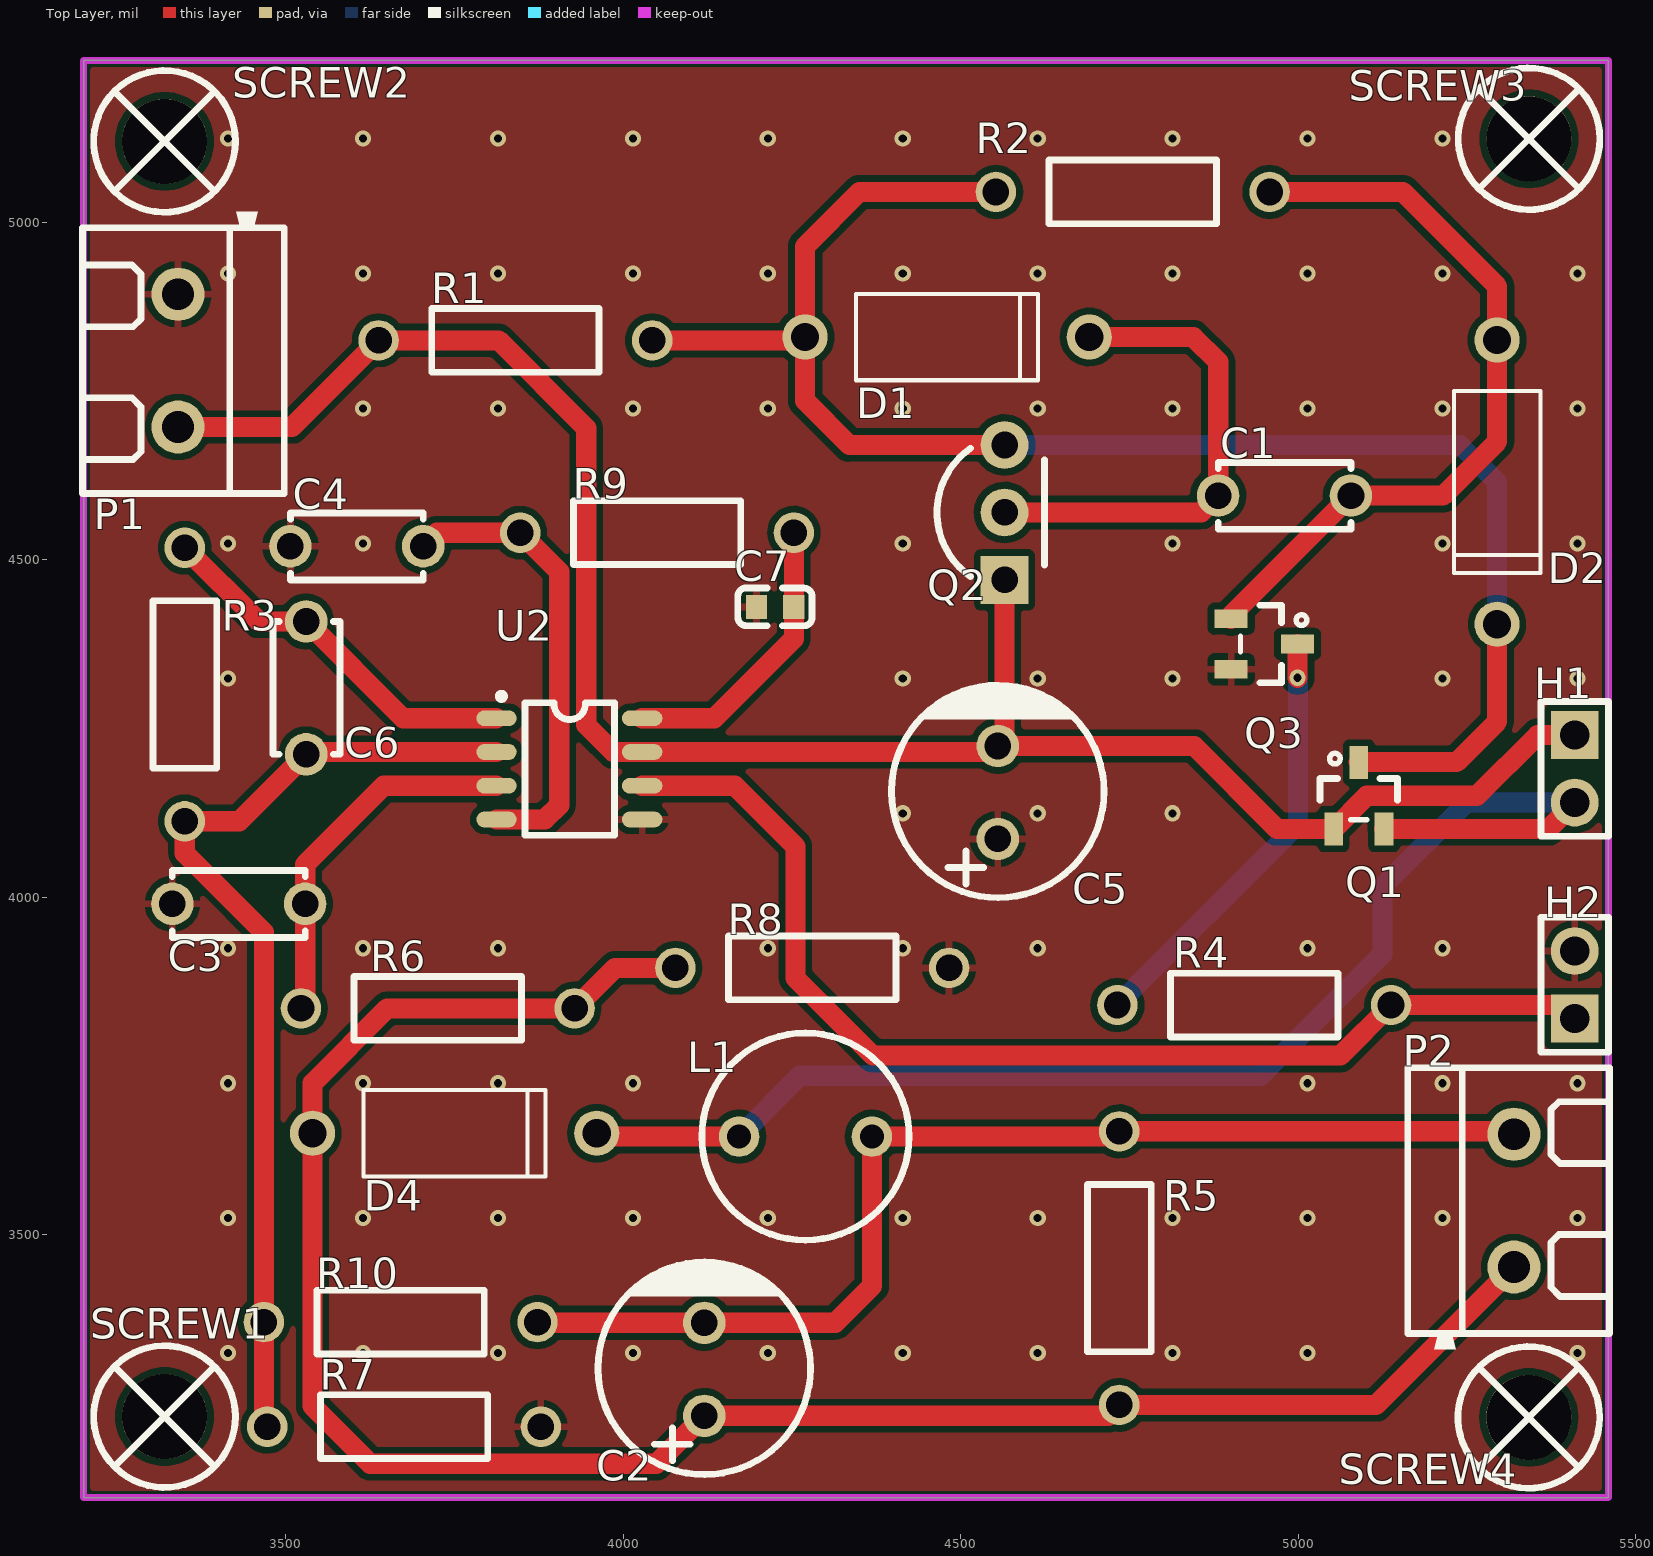
[diagram p0: Top Layer view]
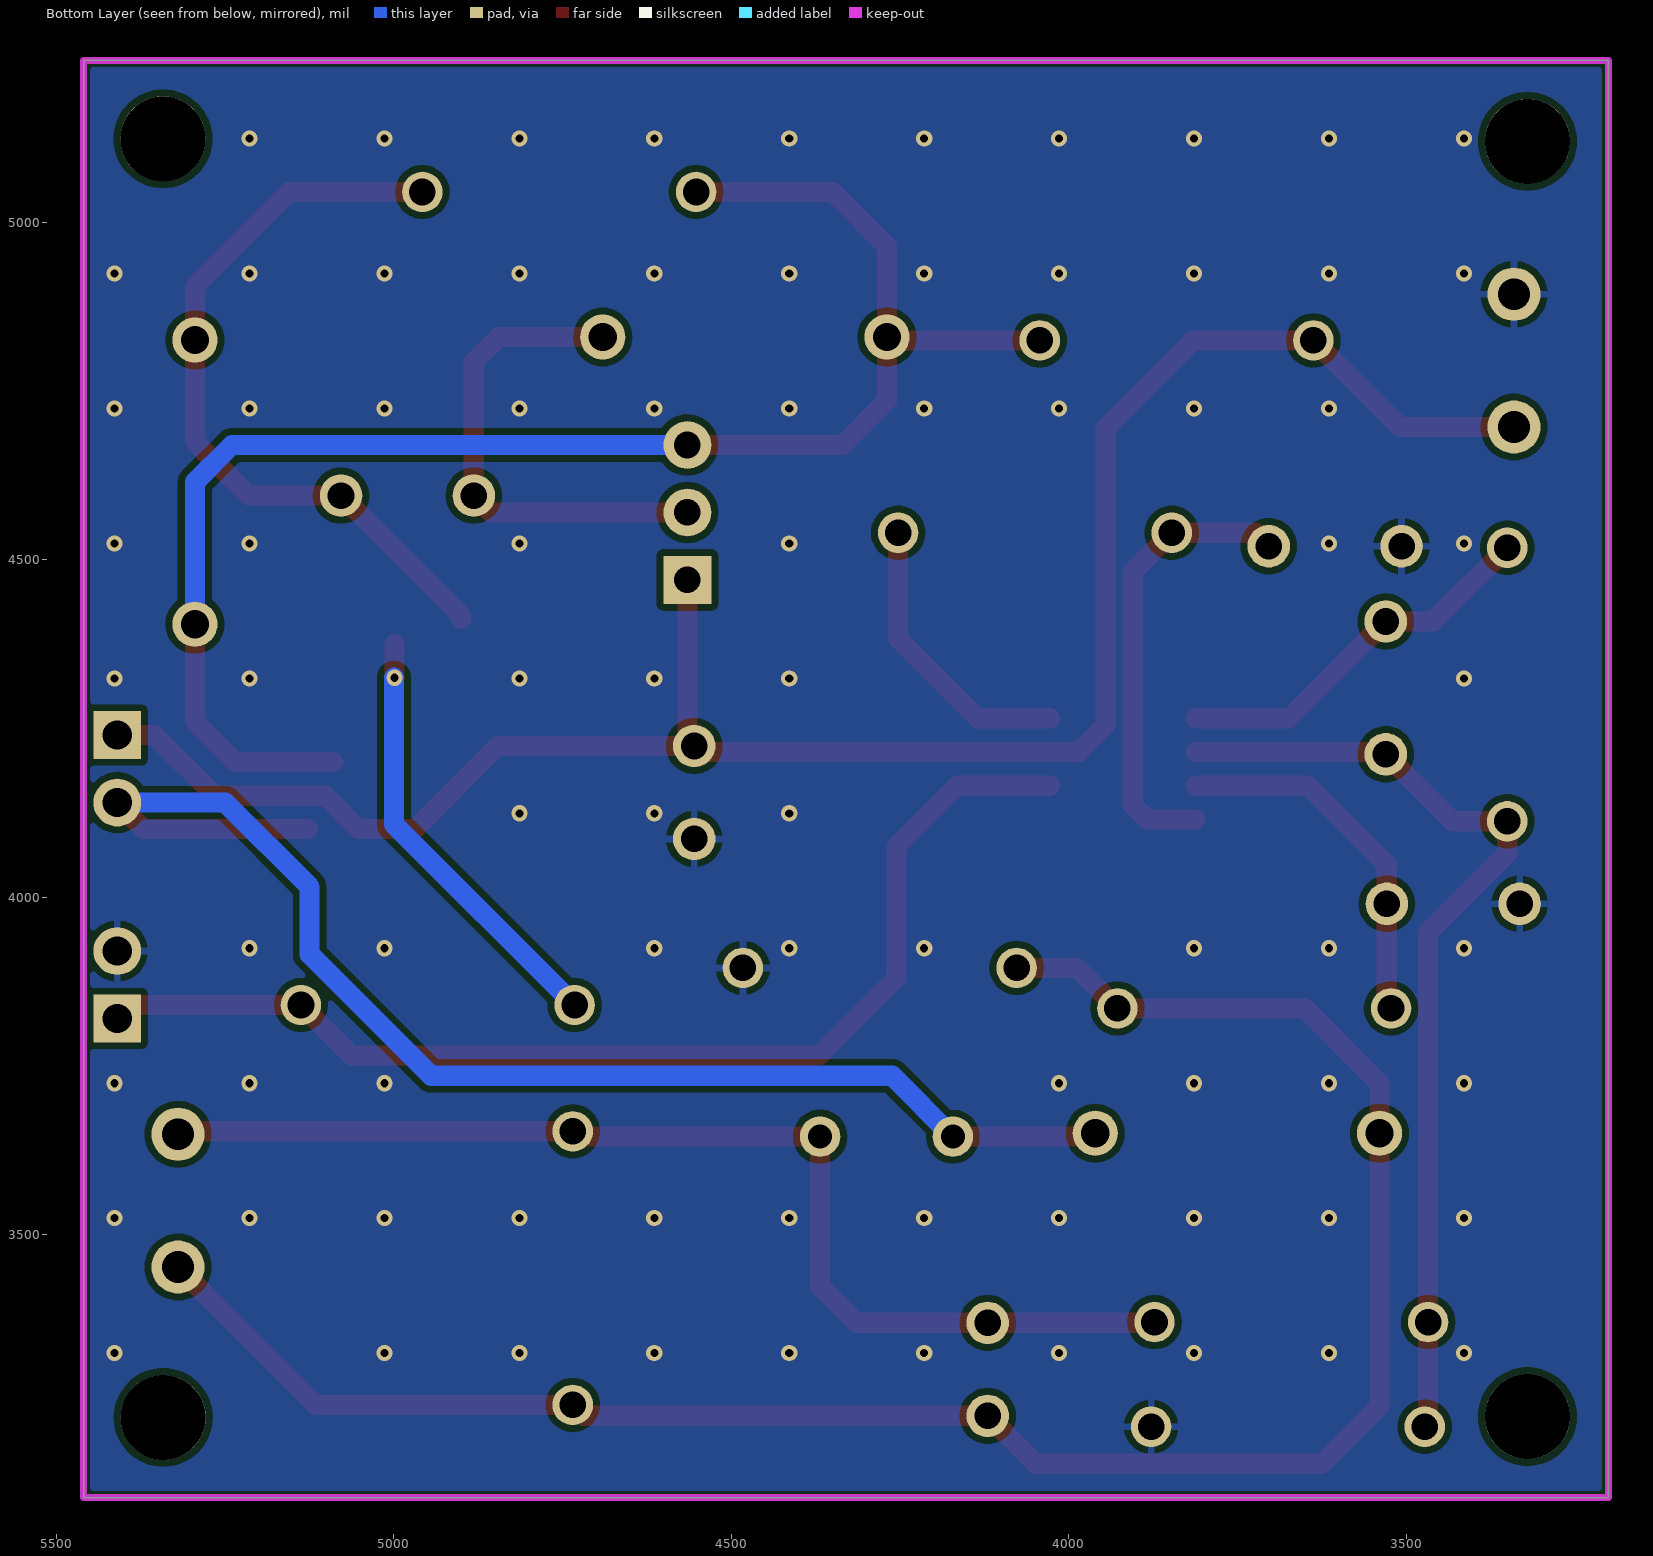
[diagram p1: Bottom Layer view, seen from below]
# Altium PCB MISC50807.pcbdoc
Units mil, origin at the board's own origin, x right, y up, seen from the top; angles counter-clockwise.
Board outline 2260 x 2130 mil, 2 copper layers (Top Layer, Bottom Layer), stack 62.206 mil thick; 33 components, 15 nets, 71 pads, 83 vias.

## Layer stack, top to bottom
Top Solder Mask Layer: solder mask 0.394, Dk 3.3
Top Layer: signal copper 1.379
Dielectric1: surface 59.449, FR4, Dk 4.5
Bottom Layer: signal copper 1.378
Bottom Solder Mask Layer: solder mask 0.394, Dk 3.3

## Board outline
3200,5240 3200,3110 5460,3110 5460,5240

## Design rules (kind name [scope] priority, off if disabled: settings)
BoardOutlineClearance copperThickness2oz_1 [All] p2 off: genericclearance=7.99 ignorepadtopadclearanceinfootprint=FALSE except(0: Arc-SplitContinuation Track-SplitContinuation SMDPad-SplitContinuation THPad-SplitContinuation Via-SplitContinuation Fill-SplitContinuation Region-SplitContinuation Poly-SplitContinuation Text-SplitContinuation Hole-SplitContinuation; 5.98: Arc-CutoutEdge SMDPad-CutoutEdge THPad-CutoutEdge Via-CutoutEdge Fill-CutoutEdge Region-CutoutEdge Text-CutoutEdge; 6.93: Hole-OutlineEdge Hole-CutoutEdge; 10: Poly-OutlineEdge Poly-CutoutEdge; 11.81: Arc-OutlineEdge Track-OutlineEdge SMDPad-OutlineEdge THPad-OutlineEdge Via-OutlineEdge Fill-OutlineEdge Region-OutlineEdge Text-OutlineEdge Track-CutoutEdge)
BoardOutlineClearance Plane_innerPlane_1 [All] p4 off: genericclearance=4.02 ignorepadtopadclearanceinfootprint=FALSE except(0: Arc-SplitContinuation Track-SplitContinuation SMDPad-SplitContinuation THPad-SplitContinuation Via-SplitContinuation Fill-SplitContinuation Region-SplitContinuation Poly-SplitContinuation Text-SplitContinuation Hole-SplitContinuation; 6: SMDPad-CutoutEdge THPad-CutoutEdge Via-CutoutEdge Fill-CutoutEdge Region-CutoutEdge Text-CutoutEdge; 6.93: Hole-OutlineEdge Hole-CutoutEdge; 10: Poly-OutlineEdge Poly-CutoutEdge; 11.8: Arc-OutlineEdge Track-OutlineEdge SMDPad-OutlineEdge THPad-OutlineEdge Via-OutlineEdge Fill-OutlineEdge Region-OutlineEdge Text-OutlineEdge; 11.81: Arc-CutoutEdge Track-CutoutEdge)
BoardOutlineClearance Copper_copperRegion_1 [All] p6 off: genericclearance=4.02 ignorepadtopadclearanceinfootprint=FALSE except(0: Arc-SplitContinuation Track-SplitContinuation SMDPad-SplitContinuation THPad-SplitContinuation Via-SplitContinuation Fill-SplitContinuation Region-SplitContinuation Poly-SplitContinuation Text-SplitContinuation Hole-SplitContinuation; 6: SMDPad-CutoutEdge THPad-CutoutEdge Via-CutoutEdge Fill-CutoutEdge Region-CutoutEdge Text-CutoutEdge; 6.93: Hole-OutlineEdge Hole-CutoutEdge; 10: Poly-OutlineEdge Poly-CutoutEdge; 11.8: Arc-OutlineEdge Track-OutlineEdge SMDPad-OutlineEdge THPad-OutlineEdge Via-OutlineEdge Fill-OutlineEdge Region-OutlineEdge Text-OutlineEdge; 11.81: Arc-CutoutEdge Track-CutoutEdge)
BoardOutlineClearance copperThickness1oz_1 [All] p8: genericclearance=4.02 ignorepadtopadclearanceinfootprint=FALSE except(0: Arc-SplitContinuation Track-SplitContinuation SMDPad-SplitContinuation THPad-SplitContinuation Via-SplitContinuation Fill-SplitContinuation Region-SplitContinuation Poly-SplitContinuation Text-SplitContinuation Hole-SplitContinuation; 6: SMDPad-CutoutEdge THPad-CutoutEdge Via-CutoutEdge Fill-CutoutEdge Region-CutoutEdge Text-CutoutEdge; 6.93: Hole-OutlineEdge Hole-CutoutEdge; 10: Poly-OutlineEdge Poly-CutoutEdge; 11.8: Arc-OutlineEdge Track-OutlineEdge SMDPad-OutlineEdge THPad-OutlineEdge Via-OutlineEdge Fill-OutlineEdge Region-OutlineEdge Text-OutlineEdge; 11.81: Arc-CutoutEdge Track-CutoutEdge)
Clearance copperThickness2oz [All] p1 off: gap=7.99 ignorepadtopadclearanceinfootprint=FALSE except(5.98: SMDPad-Track SMDPad-SMDPad THPad-Track SMDPad-THPad THPad-THPad Track-Via SMDPad-Via THPad-Via Via-Via Fill-Track Region-Track Fill-SMDPad Region-SMDPad Fill-THPad Region-THPad Fill-Via Region-Via Fill-Fill Fill-Region Region-Region Arc-Track Arc-SMDPad Arc-THPad Arc-Via Fill-Arc Region-Arc Arc-Arc Text-Track SMDPad-Text Text-THPad Text-Via Fill-Text Region-Text Arc-Text Text-Text; 6.93: Hole-Track Hole-SMDPad Hole-THPad Hole-Via Fill-Hole Region-Hole Hole-Arc Hole-Text; 10: Poly-Track Poly-SMDPad Poly-THPad Poly-Via Poly-Fill Poly-Region Poly-Poly Poly-Arc Poly-Text Poly-Hole)
Clearance Plane_innerPlane [All] p3 off: gap=4.02 ignorepadtopadclearanceinfootprint=FALSE except(5.98: SMDPad-Track SMDPad-SMDPad THPad-Track SMDPad-THPad THPad-THPad Track-Via SMDPad-Via THPad-Via Via-Via Fill-Track Region-Track Fill-SMDPad Region-SMDPad Fill-THPad Region-THPad Fill-Via Region-Via Fill-Fill Fill-Region Region-Region; 6: Arc-Track Arc-SMDPad Arc-THPad Arc-Via Fill-Arc Region-Arc Arc-Arc Text-Track SMDPad-Text Text-THPad Text-Via Fill-Text Region-Text Arc-Text Text-Text; 6.93: Hole-Track Hole-SMDPad Hole-THPad Hole-Via Fill-Hole Region-Hole Hole-Arc Hole-Text; 10: Poly-Track Poly-SMDPad Poly-THPad Poly-Via Poly-Fill Poly-Region Poly-Poly Poly-Arc Poly-Text Poly-Hole)
Clearance Copper_copperRegion [All] p5 off: gap=4.02 ignorepadtopadclearanceinfootprint=FALSE except(5.98: SMDPad-Track SMDPad-SMDPad THPad-Track SMDPad-THPad THPad-THPad Track-Via SMDPad-Via THPad-Via Via-Via Fill-Track Region-Track Fill-SMDPad Region-SMDPad Fill-THPad Region-THPad Fill-Via Region-Via Fill-Fill Fill-Region Region-Region; 6: Arc-Track Arc-SMDPad Arc-THPad Arc-Via Fill-Arc Region-Arc Arc-Arc Text-Track SMDPad-Text Text-THPad Text-Via Fill-Text Region-Text Arc-Text Text-Text; 6.93: Hole-Track Hole-SMDPad Hole-THPad Hole-Via Fill-Hole Region-Hole Hole-Arc Hole-Text; 10: Poly-Track Poly-SMDPad Poly-THPad Poly-Via Poly-Fill Poly-Region Poly-Poly Poly-Arc Poly-Text Poly-Hole)
Clearance copperThickness1oz [All] p7: gap=4.02 ignorepadtopadclearanceinfootprint=FALSE except(5.98: SMDPad-Track SMDPad-SMDPad THPad-Track SMDPad-THPad THPad-THPad Track-Via SMDPad-Via THPad-Via Via-Via Fill-Track Region-Track Fill-SMDPad Region-SMDPad Fill-THPad Region-THPad Fill-Via Region-Via Fill-Fill Fill-Region Region-Region; 6: Arc-Track Arc-SMDPad Arc-THPad Arc-Via Fill-Arc Region-Arc Arc-Arc Text-Track SMDPad-Text Text-THPad Text-Via Fill-Text Region-Text Arc-Text Text-Text; 6.93: Hole-Track Hole-SMDPad Hole-THPad Hole-Via Fill-Hole Region-Hole Hole-Arc Hole-Text; 10: Poly-Track Poly-SMDPad Poly-THPad Poly-Via Poly-Fill Poly-Region Poly-Poly Poly-Arc Poly-Text Poly-Hole)
DiffPairsRouting differentialPair [All] p1: maxlimit=6 minlimit=6 mostfreqgap=6 toplayer_minwidth=5 toplayer_prefwidth=10 toplayer_maxwidth=100 toplayer_mingap=6 toplayer_prefgap=6 toplayer_maxgap=6 bottomlayer_minwidth=5 bottomlayer_prefwidth=10 bottomlayer_maxwidth=100 bottomlayer_mingap=6 bottomlayer_prefgap=6 bottomlayer_maxgap=6 maxuncoupledlength=10
HoleToHoleClearance otherClearance [All] p1: gap=11.81 allowstackedmicrovias=TRUE
Length netLength [All] p1: minlimit=0 maxlimit=0
PasteMaskExpansion pasteMaskExpansion [All] p1: expansion=0
PlaneConnect innerPlane [All] p1: planeconnectstyle=Relief reliefexpansion=20 reliefentries=4 reliefconductorwidth=10 reliefairgap=10
PolygonConnect copperRegion [All] p1: connectstyle=Relief reliefconductorwidth=10 reliefentries=4 polygonreliefangle="90 Angle" airgapwidth=10 via.connectstyle=Relief via.reliefconductorwidth=10 via.reliefentries=4 via.polygonreliefangle="90 Angle" via.airgapwidth=10
RoutingVias viaSize [All] p1: holewidth=12.01 width=24.02 viastyle="Through Hole" minholewidth=11.81 minwidth=19.68 maxholewidth=248.03 maxwidth=393.7
SolderMaskExpansion solderMaskExpansion [IsVia] p1: expansion=-1000 istentingtop=TRUE
SolderMaskExpansion solderMaskExpansion [All] p2: expansion=2 istentingtop=FALSE
Width copperThickness2oz_2 [All] p1 off: maxlimit=100 minlimit=8 preferedwidth=10
Width copperThickness1oz_2 [All] p2: maxlimit=100 minlimit=5 preferedwidth=10

## Components (designator, comment, footprint, x,y, rotation, side; value= is the part's Value field where it differs from the comment)
C1 "1000pF" CAP-TH_L5.0-W2.5-P5.00-D1.0 4980,4595 r0 top
C2 "100uF" CAP-TH_BD8.0-P3.50-D0.6-FD_1 4120,3300 r90 top
C3 "470pF" CAP-TH_L5.0-W2.5-P5.00-D1.0 3430,3990 r0 top
C4 "4.7nF" CAP-TH_L5.0-W2.5-P5.00-D1.0 3605,4520 r0 top
C5 "100uF" CAP-TH_BD8.0-P3.50-D0.6-FD_1 4555,4155 r90 top
C6 "10nF" CAP-TH_L5.0-W2.5-P5.00-D1.0 3530,4310 r90 top
C7 "10nF" C0603 4225,4430 r0 top
D1 "SS34" DO-15_BD3.1-L6.7-P10.70-D0.8-RD 4480,4830 r180 top
D2 "1N5341BRLG" DO-15_BD3.1-L6.7-P10.70-D0.8-RD 5295,4615 r90 top
D4 "SS34" DO-15_BD3.1-L6.7-P10.70-D0.8-RD 3750,3650 r180 top
H1 "" HDR-TH_2P-P2.54-V-M-1 5410,4190 r270 top
H2 "" HDR-TH_2P-P2.54-V-M-1 5410,3870 r90 top
L1 "33uH" IND-TH_BD7.8-P5.00-D0.7 4270,3645 r0 top
P1 "KF301-2P terminal block" CONN-TH_XY301V-A-5.0-2P 3340,4795 r90 top
P2 "KF301-2P terminal block" CONN-TH_XY301V-A-5.0-2P 5320,3550 r270 top
Q1 "AOD4185" SOT-23-3_L2.9-W1.3-P1.90-LS2.4-L 5090,4150 r270 top
Q2 "BC33725TA" TO-92-3_L4.9-W3.7-P2.54-L 4565,4570 r90 top
Q3 "SI2302DS" SOT-23-3_L2.9-W1.3-P1.90-LS2.4-L 4950,4375 r180 top
R1 "300" Res_1/4W 3840,4825 r0 top
R2 "200" Res_1/4W 4755,5045 r0 top
R3 "4.7K" Res_1/4W 3350,4315 r90 top
R4 "10" Res_1/4W 4935,3840 r0 top
R5 "2.5" Res_1/4W 4735,3450 r90 top
R6 "1K" Res_1/4W 3725,3835 r0 top
R7 "2.5K" Res_1/4W 3675,3215 r180 top
R8 "0.1" Res_1/4W 4280,3895 r180 top
R9 "2K" Res_1/4W 4050,4540 r0 top
R10 "2.5K" Res_1/4W 3670,3370 r0 top
SCREW1 "" M3螺丝 3320,3230 r0 top
SCREW2 "" M3螺丝 3320,5120 r0 top
SCREW3 "" M3螺丝 5342.32,5123.78 r0 top
SCREW4 "" M3螺丝 5342.01,3228.78 r0 top
U2 "UC3843N" SOP-8_L5.1-W3.9-P1.27-LS6.0-BL 3920,4190 r270 top

## Footprints (in the part's own frame and the unit in brackets; to place one, negate y for a bottom-side part, rotate by r counter-clockwise, add the part's x,y. Pads: shape width x height; smd on the part's side, far side on the other; paste and mask are expansions set on the pad)
C0603 [mm]
  rect 0.8x0.9 smd: 1(-0.7,0) 2(0.7,0)
  silkscreen extent -1.41,-0.71 1.39,0.72
CAP-TH_BD8.0-P3.50-D0.6-FD_1 [mm]
  round 1.6 hole 1: 1(-1.75,0) 2(1.75,0)
  silkscreen extent -3.96,-4 4.04,4
CAP-TH_L5.0-W2.5-P5.00-D1.0 [mm]
  round 1.6 hole 1: 1(-2.5,0) 2(2.5,0)
  silkscreen extent -2.5,-1.27 2.5,1.25
CONN-TH_XY301V-A-5.0-2P [mm]
  round 2 hole 1.2: 1(-2.5,0) 2(2.5,0)
  silkscreen extent -5,-4 5.6,3.6
DO-15_BD3.1-L6.7-P10.70-D0.8-RD [mm]
  round 1.7 hole 1.06: 1(-5.35,0) 2(5.35,0)
  silkscreen extent -3.43,-1.63 3.43,1.63
HDR-TH_2P-P2.54-V-M-1 [mm]
  rect 1.8x1.8 hole 1.1: 1(-1.27,0)
  round 1.8 hole 1.1: 2(1.27,0)
  silkscreen extent -2.54,-1.27 2.54,1.27
IND-TH_BD7.8-P5.00-D0.7 [mil]
  round 60 hole 36: 1(-98.43,0) 2(98.42,0)
  silkscreen extent -154,-154 154,154
M3螺丝 [mil]
  round 126 hole 126 paste+0 mask+4: 1(0,0)
  silkscreen extent -105,-105 105,105
Res_1/4W [mil]
  round 60 hole 39.37 paste+0 mask+2: 1(-202.76,0) 2(202.76,0)
  silkscreen extent -124,-47 124,47
SOP-8_L5.1-W3.9-P1.27-LS6.0-BL [mm]
  oval 0.6x1.52 smd: 1(-1.905,-2.74) 2(-0.635,-2.74) 3(0.635,-2.74) 4(1.905,-2.74) 5(1.905,2.74) 6(0.635,2.74) 7(-0.635,2.74) 8(-1.905,2.74)
  silkscreen extent -2.85,-2.68 2.5,1.7
SOT-23-3_L2.9-W1.3-P1.90-LS2.4-L [mm]
  rect 1.25x0.7 smd: 1(-1.25,0) 2(1.25,0.95) 3(1.25,-0.95)
  silkscreen extent -1.6,-1.46 0.9,1.46
TO-92-3_L4.9-W3.7-P2.54-L [mm]
  rect 1.8x1.8 hole 1: 1(-2.54,0)
  round 1.8 hole 1: 2(0,0) 3(2.54,0)
  silkscreen extent -2.41,-1.5 2.41,2.54

## Via types
v1: diameter 24.02, hole 12, Top Layer to Bottom Layer, 83 vias

## Nets (pads, with @x,y where several pads share a name; then routed paths per layer and width w, separated by ;. In a path a pad name is that pad's centre, name@x,y a point inside that pad or via, vN(x,y) a via of type N, cw(c..) or ccw(c..) an arc to the next point about the centre after c; other vN are vias at no path point)
$1N5: C1.2 D2.2 Q3.3 R2.2 | length 1131.1
  Top Layer w30: Q3.3 4900.8,4417.38 C1.2 5215,4595 5295,4675 D2.2 5295,4905 5155,5045 R2.2
$1N6: C1.1 D1.1 Q2.2 | length 731.5
  Top Layer w30: Q2.2 4856.57,4570 C1.1 4881.57,4793.43 4845,4830 D1.1
$1N12: C2.1 D4.2 P2.2 R5.1 R6.2 R8.2 | length 3024.2
  Top Layer w30: R8.2 3987.76,3895 R6.2 3650,3835 3539.37,3724.37 D4.2 3539.37,3245.63 3625,3160 4048.9,3160 C2.1 4718.86,3231.1 R5.1 5115.66,3247.24 P2.2
$1N13: C2.2 L1.2 P2.1 R5.2 R10.2 | length 1696.9
  Top Layer w30: R10.2 3873.86,3368.9 C2.2 4313.9,3368.9 4368.43,3423.43 L1.2 4727.24,3645 R5.2 5315.66,3652.76 P2.1
$1N14: C6.1 R3.1 R7.2 R10.1 U2.2 | length 1452.6
  Top Layer w30: R7.2 3467.24,3220 R10.1 3467.24,3947.76 3350,4065 R3.1 3430.66,4112.24 C6.1 3533.42,4215 U2.2
$1N15: C6.2 R3.2 U2.1 | length 566.8
  Top Layer w30: R3.2 3459.34,4408.43 C6.2 3673.43,4265 U2.1
$1N18: C4.2 R9.1 U2.4 | length 681.5
  Top Layer w30: C4.2 3723.43,4540 R9.1 3905,4482.24 3905,4136.21 3883.79,4115 U2.4
$1N19: C7.2 R9.2 U2.8 | length 430.9
  Top Layer w30: U2.8 4135,4265 4252.76,4382.76 R9.2
$1N20: C3.2 R6.1 U2.3 | length 548
  Top Layer w30: R6.1 3528.43,3841.18 C3.2 3528.43,4048.43 3645,4165 U2.3
$1N23: D1.2 D2.1 Q1.1 Q2.3 R1.2 R2.1 | length 2434.1
  Top Layer w30: R1.2 4264.37,4825 D1.2 ; R2.1 4350,5045 4269.37,4964.37 D1.2 ; Q2.3 4335,4670 4269.37,4735.63 D1.2 ; Q1.1@5090,4200 5235,4200 5295,4260 D2.1
  Bottom Layer w30: Q2.3 5240,4670 5295,4615 D2.1
$1N24: D4.1 H1.2 L1.1 Q1.2 | length 2013.9
  Top Layer w30: D4.1 3965.63,3645 L1.1 ; Q1.2 5370.8,4100.8 H1.2
  Bottom Layer w30: L1.1 4261.57,3735 4945,3735 5125,3915 5125,4015 5250,4140 H1.2
$1N27: Q3.1 R4.1 | length 645.9
  Top Layer w30: v1(4999.2,4325) Q3.1
  Bottom Layer w30: R4.1 5000,4107.76 v1@5000,4325
$1N28: H2.1 R4.2 U2.6 | length 1701.4
  Top Layer w30: U2.6 4165,4165 4255,4075 4255,3880 4370,3765 5062.76,3765 R4.2 5390,3840 H2.1
+15V: C5.2 H1.1 P1.1 Q1.3 Q2.1 R1.1 U2.7 | length 2996.2
  Top Layer w30: P1.1 3508.82,4696.57 R1.1 3815,4825 3945,4695 3945,4255 3985,4215 U2.7 4546.1,4215 C5.2 ; Q2.1 4565,4233.9 C5.2 ; H1.1 5355,4240 5265,4150 5101.8,4150 Q1.3 4969.2,4100.8 4846.1,4223.9 C5.2
GND: C3.1 C4.1 C5.1 C7.1 H2.2 P1.2 Q3.2 R7.1 R8.1 U2.5
  other v1: 3414.1,3324.1 3614.1,3324.1 3814.1,3324.1 4014.1,3324.1 4214.1,3324.1 4414.1,3324.1 4614.1,3324.1 4814.1,3324.1 5014.1,3324.1 5414.1,3324.1 3414.1,3524.1 3614.1,3524.1 3814.1,3524.1 4014.1,3524.1 4214.1,3524.1 4414.1,3524.1 4614.1,3524.1 4814.1,3524.1 5014.1,3524.1 5214.1,3524.1 5414.1,3524.1 3414.1,3724.1 3614.1,3724.1 3814.1,3724.1 4014.1,3724.1 5014.1,3724.1 5214.1,3724.1 5414.1,3724.1 3414.1,3924.1 3614.1,3924.1 3814.1,3924.1 4214.1,3924.1 4414.1,3924.1 4614.1,3924.1 5014.1,3924.1 5214.1,3924.1 4414.1,4124.1 4614.1,4124.1 4814.1,4124.1 3414.1,4324.1 4414.1,4324.1 4614.1,4324.1 4814.1,4324.1 5214.1,4324.1 5414.1,4324.1 3414.1,4524.1 3614.1,4524.1 4414.1,4524.1 4814.1,4524.1 5214.1,4524.1 5414.1,4524.1 3614.1,4724.1 3814.1,4724.1 4014.1,4724.1 4214.1,4724.1 4414.1,4724.1 4614.1,4724.1 4814.1,4724.1 5014.1,4724.1 5214.1,4724.1 5414.1,4724.1 3414.1,4924.1 3614.1,4924.1 3814.1,4924.1 4014.1,4924.1 4214.1,4924.1 4414.1,4924.1 4614.1,4924.1 4814.1,4924.1 5014.1,4924.1 5214.1,4924.1 5414.1,4924.1 3414.1,5124.1 3614.1,5124.1 3814.1,5124.1 4014.1,5124.1 4214.1,5124.1 4414.1,5124.1 4614.1,5124.1 4814.1,5124.1 5014.1,5124.1 5214.1,5124.1
pads on no net: SCREW1.1 SCREW2.1 SCREW3.1 SCREW4.1

## Polygon pours and split planes (outlines as drawn)
GND on Top Layer (solid, remove dead copper, pour order 0): 3000,5315 3000,3000 5765,3000 5765,5315
GND on Bottom Layer (solid, remove dead copper, pour order 2): 3100,5285 3100,3040 5595,3040 5595,5285

## Keep-outs
Board Outline Layer:
  the board outline again, w10